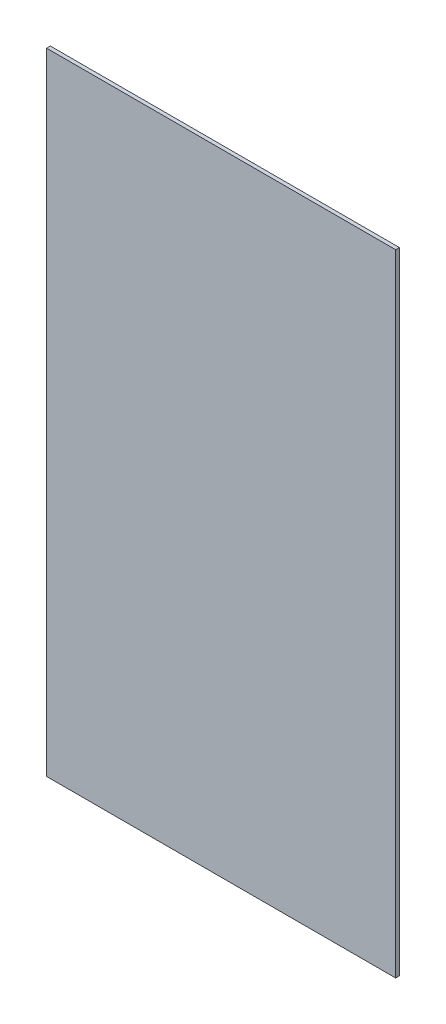
from build123d import *

# Parameters (mm, degrees)
SKETCH_1_W      = 466
SKETCH_1_H      = 842
EXTRUDE_1_DEPTH = 5


with BuildPart() as part:
    # 草图1 → 凸台-拉伸1 (new body)
    with BuildSketch(Plane.XY):
        Rectangle(SKETCH_1_W, SKETCH_1_H)
    extrude(amount=EXTRUDE_1_DEPTH)


solid = part.part
